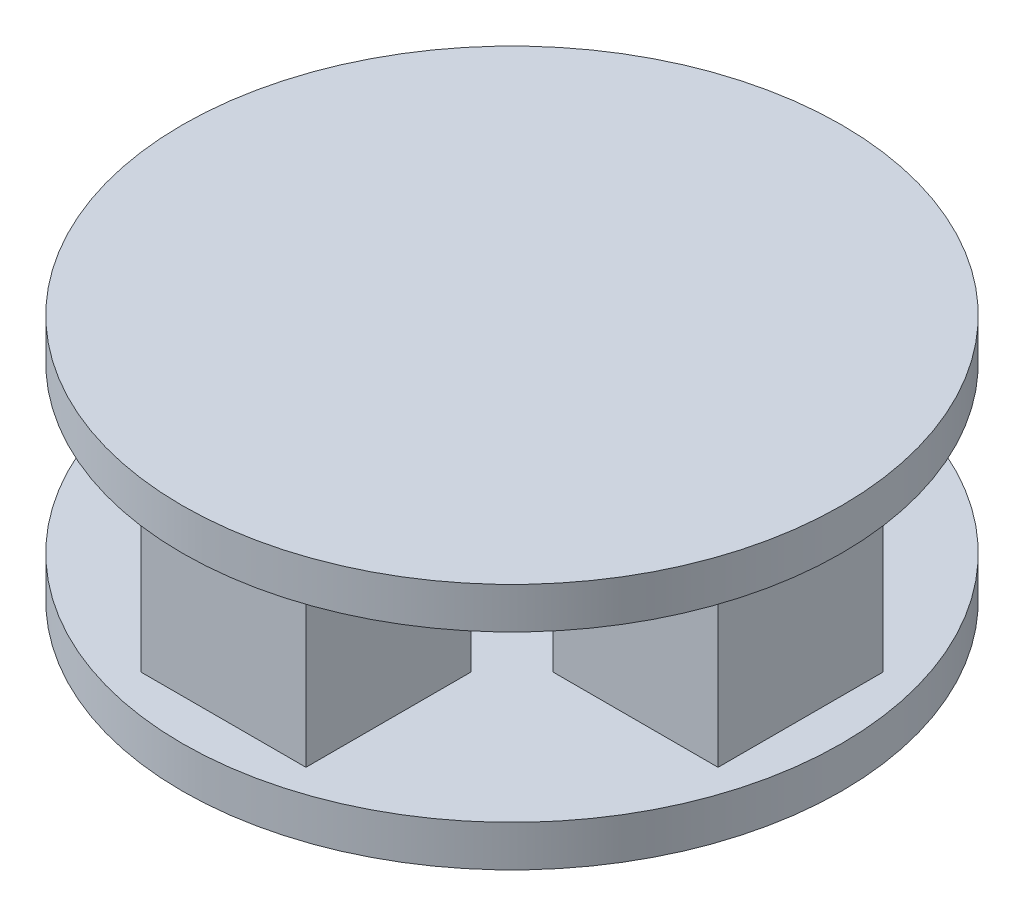
SolidWorks part; units mm, degrees
ref_plane "Front Plane" through (0, 0, 0) normal (0, 0, 1) x (1, 0, 0)
ref_plane "Top Plane" through (0, 0, 0) normal (0, 1, 0) x (1, 0, 0)
ref_plane "Right Plane" through (0, 0, 0) normal (1, 0, 0) x (0, 0, -1)
other "Configuration Table"
sketch "Sketch1" plane through (0, 0, 0) normal (0, 1, 0) x (1, 0, 0)
  circle A0 centre (0, 0) radius 16
  dimension "D1" = 32
extrude "Boss-Extrude2" add sketch "Sketch1" along normal blind 2
sketch "Sketch4" plane through (0, 2, 0) normal (0, 1, 0) x (1, 0, 0)
  line L1 (-6, 4) -> (-14, 4)
  line L2 (-4, -6) -> (4, -6)
  line L3 (-4, -6) -> (-4, -14)
  line L4 (-4, -14) -> (4, -14)
  line L5 (4, -6) -> (4, -14)
  line L6 (-4, -6) -> (4, -14) construction
  line L7 (-4, -14) -> (4, -6) construction
  line L8 (-6, 4) -> (-6, -4)
  line L9 (-6, -4) -> (-14, -4)
  line L10 (-14, 4) -> (-14, -4)
  line L11 (4, 6) -> (4, 14)
  line L12 (4, 6) -> (-4, 6)
  line L13 (-4, 6) -> (-4, 14)
  line L14 (4, 14) -> (-4, 14)
  line L15 (6, -4) -> (14, -4)
  line L16 (6, -4) -> (6, 4)
  line L17 (6, 4) -> (14, 4)
  line L18 (14, -4) -> (14, 4)
  point P22 (0, 0)
  dimension "D2" = 8
  dimension "D3" = 8
  dimension "D4" = 4
extrude "Boss-Extrude7" add sketch "Sketch4" along normal blind 8
ref_plane "Plane4" through (0, 10, 0) normal (0, -1, 0) x (-1, 0, 0)
sketch "Sketch5" plane through (0, 10, 0) normal (0, -1, 0) x (-1, 0, 0)
  circle A0 centre (0, 0) radius 16
  dimension "D1" = 32
extrude "Boss-Extrude8" add sketch "Sketch5" against normal blind 2
